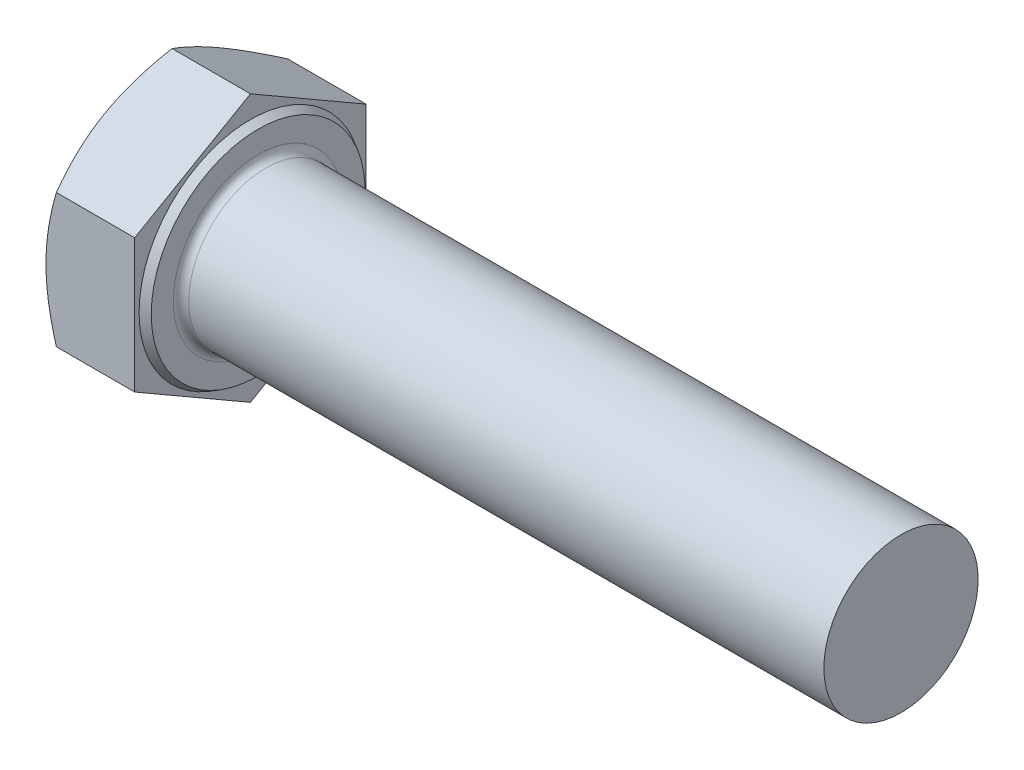
SolidWorks part; units mm, degrees
ref_plane "前视" through (0, 0, 0) normal (0, 0, 1) x (1, 0, 0)
ref_plane "上视" through (0, 0, 0) normal (0, 1, 0) x (1, 0, 0)
ref_plane "右视" through (0, 0, 0) normal (1, 0, 0) x (0, 0, -1)
sketch "草图1" plane through (0, 0, 0) normal (1, 0, 0) x (0, 0, -1)
  line L0 (9, 5.1962) -> (9, -5.1962)
  line L1 (-9, 5.1962) -> (-9, -5.1962)
  line L2 (9, -5.1962) -> (0, -10.3923)
  line L3 (0, -10.3923) -> (-9, -5.1962)
  line L4 (9, 5.1962) -> (0, 10.3923)
  line L5 (0, 10.3923) -> (-9, 5.1962)
  circle A0 centre (0, 0) radius 10.015 construction
  dimension "e" = 20.03
  dimension "s" = 18
  dimension "D2" = 120
  dimension "D3" = 9
  dimension "D4" = 9
  dimension "D5" = 9
extrude "基体-拉伸" add sketch "草图1" along normal blind 7.5
sketch "草图2" plane through (0, 0, 0) normal (0, 0, 1) x (1, 0, 0)
  line L0 (0, 5.1962) -> (0, -5.1962) construction
  line L1 (0, 0) -> (57.5, 0)
  line L2 (0, 0) -> (0, 6)
  line L3 (0, 6) -> (27.5, 6)
  line L4 (57.5, 0) -> (57.5, 4.4845)
  line L5 (7.5, 10.3923) -> (7.5, 5.1962) construction
  line L7 (0, 0) -> (69.5, 0) construction
  line L8 (57.5, -4.4845) -> (27.5, -6) construction
  line L9 (0, -6) -> (27.5, -6) construction
  line L10 (9.25, 6) -> (9.25, 0) construction
  line L11 (27.5, 15.24) -> (27.5, -1.27) construction
  line L12 (7.5, 5.1962) -> (7.5, -5.1962) construction
  line L13 (27.5, 6) -> (57.5, 6)
  line L14 (57.5, 6) -> (57.5, 4.4845)
  dimension "l" = 50
  dimension "d" = 12
  dimension "Minor_dia" = 8.969
  dimension "p" = 1.75
  dimension "b" = 30
  dimension "ds" = 12
revolve "凸台-旋转1" add sketch "草图2" angle 360 about L7
cosmetic thread "螺旋线1" parameters "Thread_length"=30, "Thread_minor"=8.969
sketch "草图3" plane through (0, 0, 0) normal (0, 0, 1) x (1, 0, 0)
  line L0 (0, 9) -> (3.6906, 15.3923)
  line L1 (0, 10.3923) -> (0, 5.1962) construction
  line L2 (3.6906, 15.3923) -> (3.6906, 20.3923)
  line L3 (3.6906, 20.3923) -> (-10, 20.3923)
  line L4 (-10, 20.3923) -> (-10, 9)
  line L5 (-10, 9) -> (0, 9)
  line L6 (0, 0) -> (99.06, 0) construction
  line L7 (7.5, 10.3923) -> (0, 10.3923) construction
  dimension "D1" = 9
  dimension "D2" = 5
  dimension "D3" = 10
  dimension "D4" = 5
  dimension "Head_ch_ang" = 30
revolve "切除-旋转1" cut sketch "草图3" angle 360 about L6
sketch "草图4" plane through (0, 0, 0) normal (0, 0, 1) x (1, 0, 0)
  line L0 (7.5, 0) -> (7.5, 8.315) construction
  line L2 (7.5, -6) -> (7.5, 6) construction
  line L3 (7.5, 10.3923) -> (7.5, 5.1962) construction
  line L4 (7.5, 8.315) -> (6.9, 8.6614)
  line L5 (0, 0) -> (95.25, 0) construction
  line L6 (0, 0) -> (69.5, 0) construction
  line L9 (6.9, 8.6614) -> (6.9, 10.3923)
  line L10 (7.5, 10.3923) -> (0.8038, 10.3923) construction
  line L11 (6.9, 10.3923) -> (7.5, 10.3923)
  line L12 (7.5, 10.3923) -> (7.5, 8.315)
  dimension "D1" = 120
  dimension "c" = 0.6
  dimension "dw" = 16.63
revolve "切除-旋转3" cut sketch "草图4" angle 360 about L5
fillet "圆角" radius 0.6 1 edges at (7.5, 0, -6)
sketch "草图6" plane through (0, 0, 0) normal (0, 0, 1) x (1, 0, 0)
  line L0 (0, 0) -> (57.5, 0) construction
  line L1 (57.5, -6) -> (57.5, 6) construction
  line L2 (57.5, 0) -> (57.5, 6) construction
  line L4 (56.625, 6) -> (58.375, 6)
  line L5 (56.625, 6) -> (57.5, 4.4845)
  line L6 (57.5, 4.4845) -> (58.375, 6)
  dimension "D1" = 1.75
revolve "切除-旋转4" [suppressed] cut sketch "草图6" angle 360 about L0
pattern_linear "阵列(线性)1" [suppressed]
